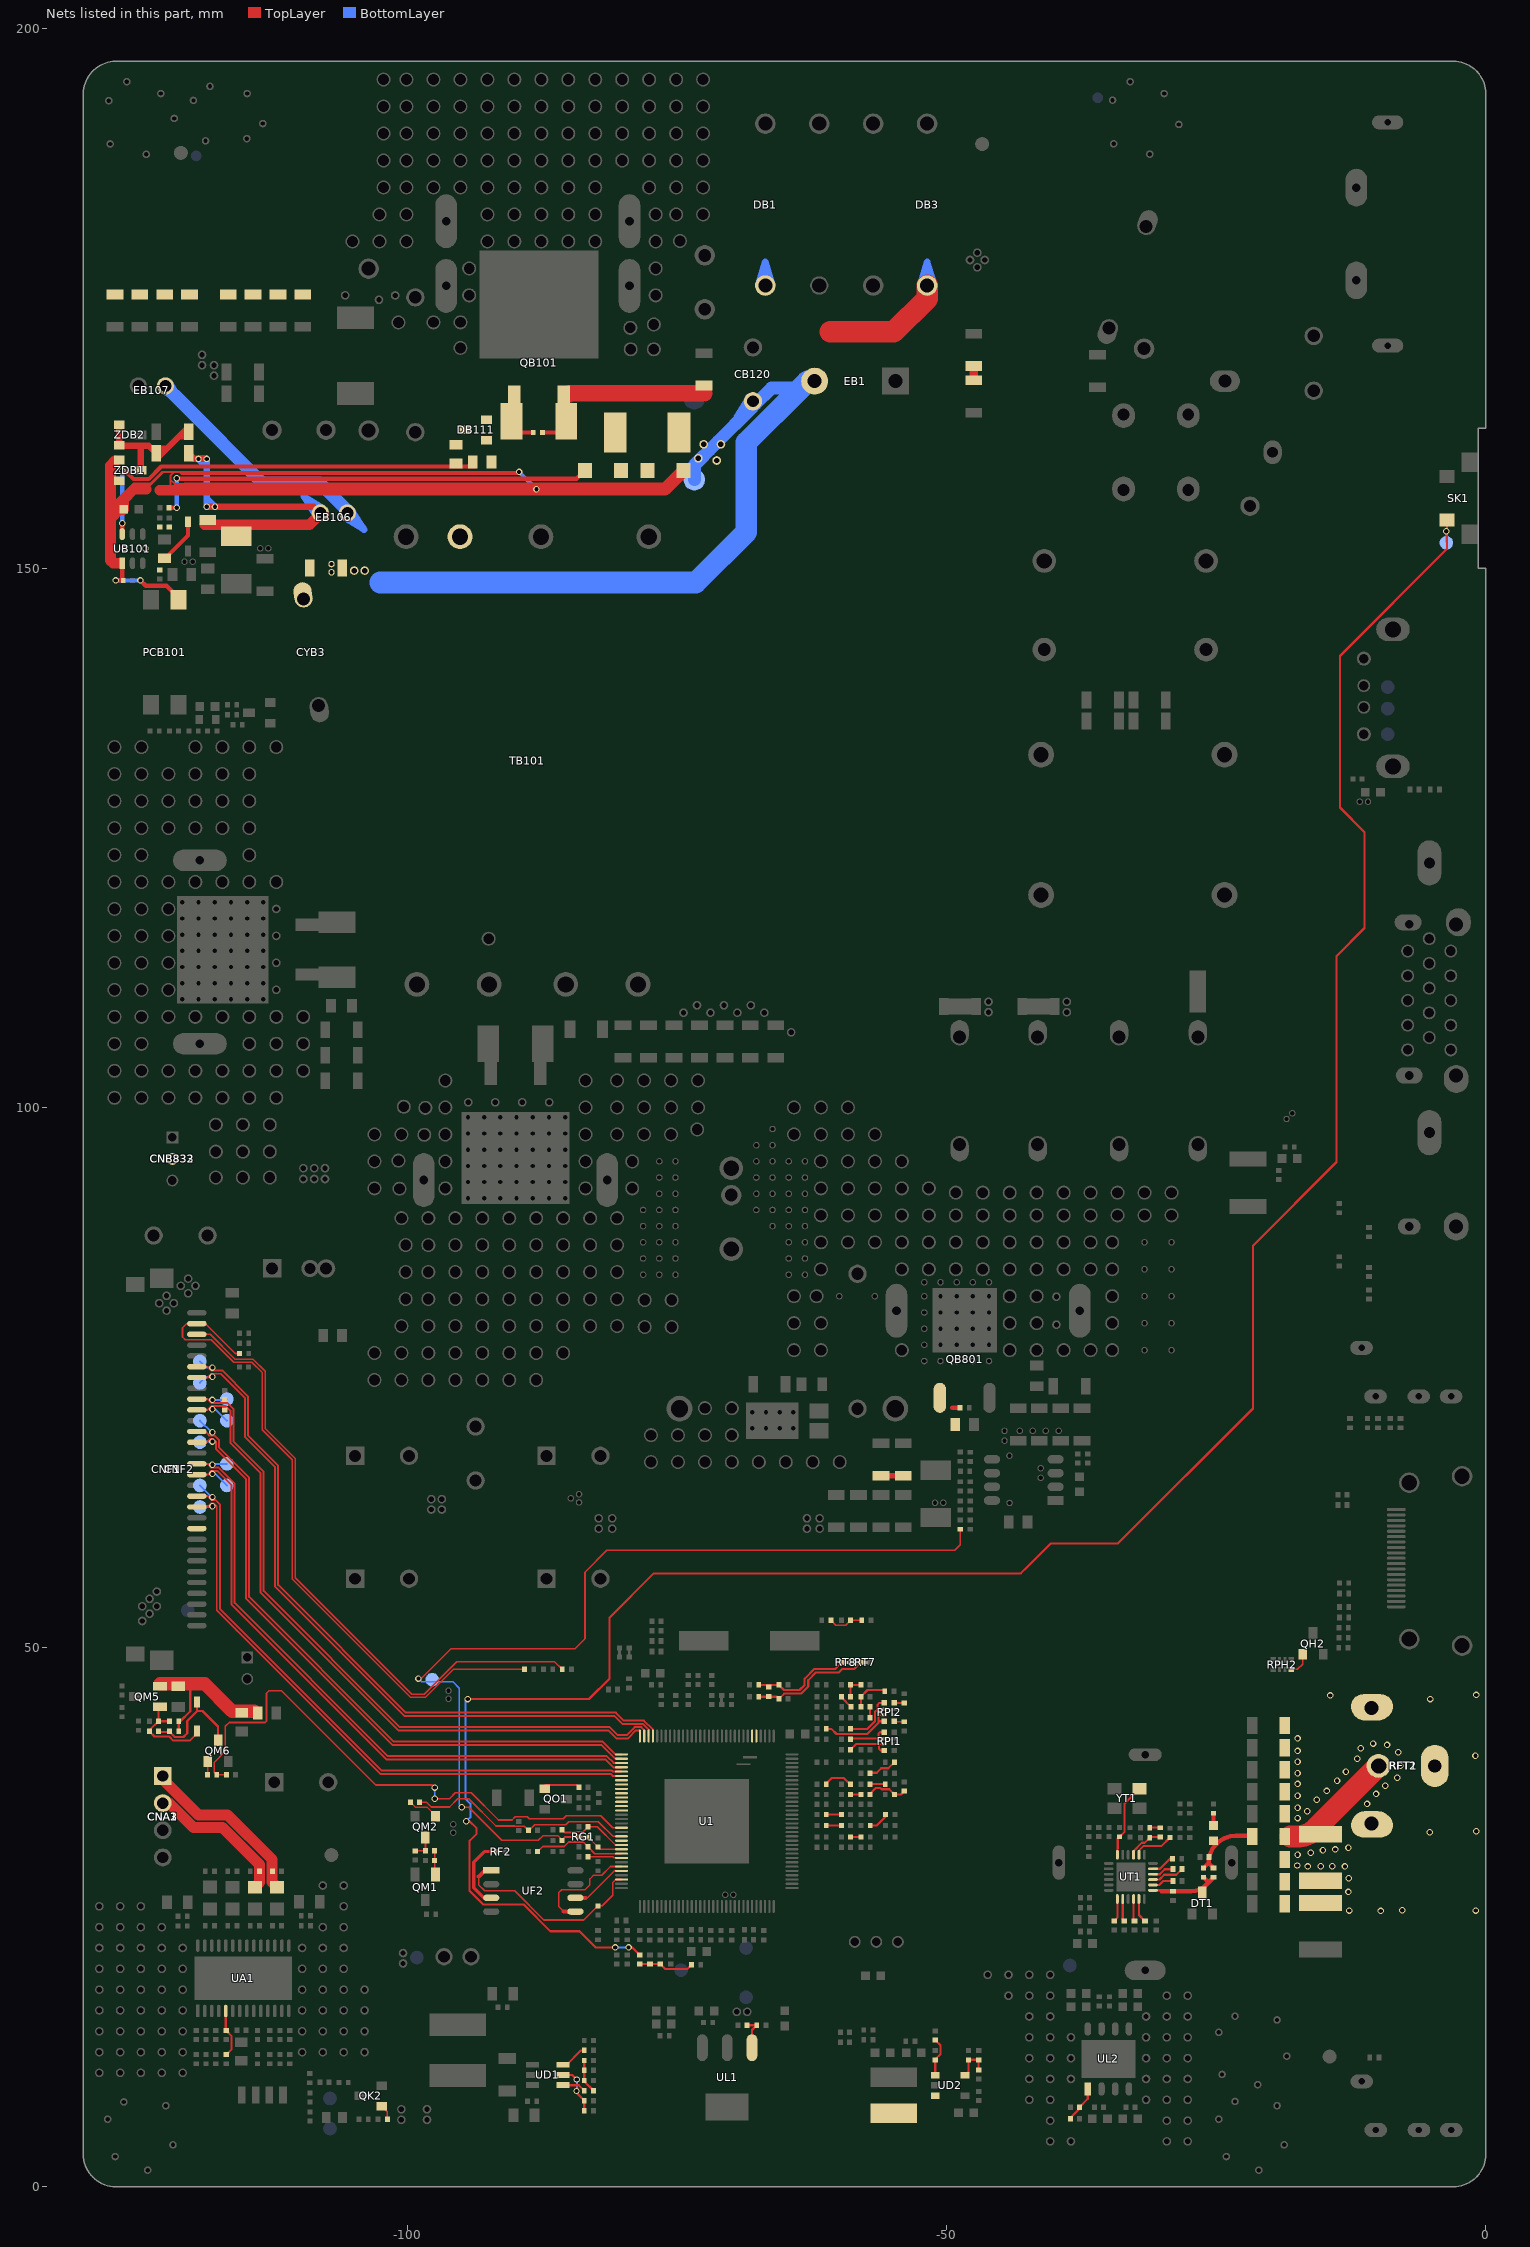
[diagram p0: the nets of this part, all layers, seen from the top]
# Altium PCB MISC84438.PcbDoc (part 12 of 15)
Units mm, origin at the board's own origin, x right, y up, seen from the top; angles counter-clockwise.
Board outline 130 x 197 mm, 2 copper layers (TopLayer, BottomLayer), stack 1.571 mm thick; 574 components, 314 nets, 2636 pads, 811 vias.

## Via types
v1: diameter 0.6, hole 0.4, TopLayer to BottomLayer, tented both sides, 780 vias
v2: diameter 0.7, hole 0.5, TopLayer to BottomLayer, tented both sides, 15 vias
v3: diameter 0.8, hole 0.6, TopLayer to BottomLayer, tented both sides, 12 vias
v4: diameter 0.8, hole 0.5, TopLayer to BottomLayer, tented both sides, 4 vias

## Nets (pads, with @x,y where several pads share a name; then routed paths per layer and width w, separated by ;. In a path a pad name is that pad's centre, name@x,y a point inside that pad or via, vN(x,y) a via of type N, cw(c..) or ccw(c..) an arc to the next point about the centre after c; other vN are vias at no path point) (continued)
NetCD13_2: CD13.2 RD6.1 RD7.2 UD2.5 | length 3.4
  TopLayer w0.203: UD2.5@-48.28,10.335 -47.955,10.66 CD13.2@-47.955,11.754 RD6.1@-47.015,11.754 RD7.2@-47.015,10.814
NetCD17_2: CD17.2 RD8.2 UD2.1 | length 3.7
  TopLayer w0.203: UD2.1@-51.03,10.335 -51.03,11.751 CD17.2@-51.027,11.754 ; RD8.2@-51.027,13.583 -50.548,13.104 -50.548,12.285 -51.027,11.806 CD17.2@-51.027,11.754 ; CD17.2@-50.933,11.754 CD17.2@-51.027,11.754
NetCD20_2: CD20.2 RD13.1 RD15.2 RD16.2 | length 3.1
  TopLayer w0.203: CD20.2@-83.571,11.697 RD13.1@-83.571,10.771 RD16.2@-83.571,9.842 -83.571,9.753 RD15.2@-82.721,8.903
NetCF26_2: CF26.2 RF12.1 | length 2.7
  TopLayer w0.203: CF26.2@-57.081,38.303 -57.014,38.37 -56.464,38.37 -56.052,38.782 -55.383,38.782 RF12.1@-54.82,39.345
NetCF31_2: CF31.2 RF16.1 | length 2
  TopLayer w0.203: CF31.2@-57.055,33.477 -56.464,33.477 -55.632,34.309 RF16.1@-55.632,34.493
NetCF34_1: CF34.1 RF19.2 | length 2.8
  TopLayer w0.203: CF34.1@-61.145,37.312 -61.145,37.369 -60.63,37.883 -59.506,37.883 -58.936,37.313 RF19.2@-58.884,37.313
NetCF39_2: CF39.2 CF40.2 RF24.1 | length 3.2
  TopLayer w0.152: RF24.1@-60.7,52.489 -60.247,52.036 -59.337,52.036 CF39.2@-58.884,52.489 CF40.2@-57.854,52.489
NetCI1_2: CI1.2 RI2.2 | length 1
  TopLayer w0.203: CI1.2@-58.884,36.347 RI2.2@-57.931,36.346
NetCI3_2: CI3.2 RPI2.5 RPI2.7 | length 7.4
  TopLayer w0.198: CI3.2@-61.145,42.431 -60.661,42.431 -60.185,41.955 -59.931,41.955 -57.331,41.955 -56.304,42.981 -56.304,43.167 ; RPI2.7@-55.695,43.143 RPI2.7@-55.746,43.143 -56.28,43.143 -56.304,43.167 ; RPI2.5@-55.695,43.743 RPI2.5@-55.746,43.743 -56.232,43.743 -56.304,43.67 -56.304,43.167
NetCI4_2: CI4.2 RPI2.1 RPI2.3 | length 5.6
  TopLayer w0.198: CI4.2@-58.884,42.431 -57.314,42.431 -56.63,43.115 -56.63,43.993 -56.38,44.243 ; RPI2.3@-55.695,44.243 -56.38,44.243 ; RPI2.1@-55.695,44.843 -56.211,44.843 -56.38,44.674 -56.38,44.243
NetCI6_2: CI6.2 RPI1.5 RPI1.7 | length 4.4
  TopLayer w0.198: CI6.2@-58.884,40.5 -58.359,41.025 -56.236,41.025 ; RPI1.7@-55.746,40.425 -56.097,40.425 -56.236,40.564 -56.236,41.025 ; RPI1.5@-55.695,41.025 RPI1.5@-55.746,41.025 -56.236,41.025
NetCI7_2: CI7.2 RPI1.1 RPI1.3 | length 4
  TopLayer w0.198: -58.621,41.525 -56.312,41.525 ; RPI1.1@-55.746,42.125 -56.173,42.125 -56.312,41.986 -56.312,41.525 ; RPI1.3@-55.695,41.525 RPI1.3@-55.746,41.525 -56.312,41.525
NetCI8_2: CI8.2 RI8.2 | length 1.4
  TopLayer w0.203: CI8.2@-57.081,37.313 RI8.2@-55.67,37.313
NetCM1_2: CM1.2 QM1.G RM2.2 | length 2.1
  TopLayer w0.152: QM1.G@-97.441,29.012 RM2.2@-97.441,31.147
NetCM3_1: CM3.1 CM7.1 DM1.K QM5.G RM7.2 | length 8.9
  TopLayer w0.203: QM5.G@-122.892,44.478 -123.032,44.338 CM7.1@-123.032,43.142 ; CM3.1@-122.003,43.142 CM7.1@-123.032,43.142 ; DM1.K@-119.344,42.124 -120.125,41.343 -121.66,41.343 -122.041,41.724 -123.403,41.724 RM7.2@-123.882,42.202 -123.882,42.292 CM7.1@-123.032,43.142
NetCNB832_2: CNB832.2 CNB833.2
NetCNF1_21: CNF1.21 CNF2.21
NetCO1_1: CO1.1 RO3.2 RO13.2 | length 3.4
  TopLayer w0.203: CO1.1@-57.931,44.475 RO3.2@-57.931,45.416 -57.317,46.029 -55.814,46.029 RO13.2@-55.721,45.936
NetCO1_2: CO1.2 RO1.2 | length 1
  TopLayer w0.198: RO1.2@-57.081,43.459 CO1.2@-57.081,44.475
NetCO4_1: CO4.1 RO7.2 RO15.2 | length 2.1
  TopLayer w0.203: CO4.1@-58.884,45.415 RO7.2@-58.884,46.507 ; RO7.2@-58.844,46.507 RO7.2@-58.884,46.507 ; RO15.2@-57.931,46.507 RO7.2@-58.884,46.507
NetCO4_2: CO4.2 RO5.2 | length 1.3
  TopLayer w0.203: CO4.2@-59.734,45.415 -59.734,45.351 RO5.2@-58.859,44.475
NetCT10_1: CT10.1 CT20.1 RT7.2 RT7.3 RT9.1 | length 11.3
  TopLayer w0.203: CT20.1@-67.4,45.415 -66.453,45.415 -65.735,45.415 CT10.1@-65.532,45.212 -65.046,45.698 -63.481,45.698 -62.814,46.364 -62.814,46.952 -62.116,47.65 -59.992,47.65 -59.666,47.977 -58.544,47.977 RT7.2@-57.931,48.59
NetCT11_2: CT11.2 UT1.20 | length 2.1
  TopLayer w0.203: UT1.20@-33.656,26.664 -33.656,24.754 CT11.2@-33.533,24.631
NetCT12_1: CT12.1 UT1.19 | length 2.2
  TopLayer w0.203: CT12.1@-34.461,24.631 -34.156,24.936 UT1.19@-34.156,26.664
NetCT13_2: CT13.2 DT1.2 LT3.2 LT6.1 UT1.1 | length 6.7
  TopLayer w0.229: UT1.1@-30.856,27.464 -30.107,27.464
  TopLayer w0.401: -30.061,27.387 LT6.1@-28.981,27.387 -27.305,27.387 ccw(c-27.305,29.288) -25.961,27.944 LT3.2@-25.227,28.678 ; CT13.2@-26.167,28.678 -25.705,28.216
NetCT15_2: CT15.2 UT1.12 YT1.3 | length 7
  TopLayer w0.203: UT1.12@-34.156,30.764 -34.156,31.304 -34.116,31.344 -34.116,32.273 CT15.2@-33.96,32.429 -33.481,32.908 -33.481,35.513 YT1.3@-32.115,36.879
NetCT17_1: CT17.1 LT9.2 | length 1.1
  TopLayer w0.401: LT9.2@-25.248,33.485 CT17.1@-25.248,34.614
NetCT21_1: CT21.1 UT1.5 | length 2.2
  TopLayer w0.203: UT1.5@-30.856,29.464 -30.2,29.464 -29.274,30.391 CT21.1@-29.038,30.391
NetCT23_1: CT23.1 CT24.2 RT8.2 RT8.3 RT9.2 | length 9.1
  TopLayer w0.203: CT23.1@-67.4,46.507 -66.453,46.507 -65.532,46.507 -65.053,46.028 -63.618,46.028 -63.144,46.501 -63.144,47.089 -62.253,47.98 -60.314,47.98 RT8.2@-59.875,48.42
NetCT25_1: CT25.1 UT1.8 | length 3.8
  TopLayer w0.191: UT1.8@-32.156,30.764 -32.156,31.149 -31.748,31.557 -30.083,31.557 CT25.1@-29.274,32.366
NetCT26_2: CT26.2 RT11.2 UT1.9 | length 3.3
  TopLayer w0.191: UT1.9@-32.656,30.764 -32.656,31.098 -31.88,31.874 -31.619,31.874 CT26.2@-31.147,32.346 -31.076,32.417 RT11.2@-30.188,32.417
NetCT29_2: CT29.2 RT11.1 | length 1
  TopLayer w0.191: CT29.2@-31.147,33.274 -30.195,33.274 RT11.1@-30.188,33.267
NetCV1_2: CV1.2 RV1.1 | length 1.4
  TopLayer w0.18: CV1.2@-61.145,34.493 RV1.1@-59.734,34.493
NetCV3_2: CV3.2 RV3.1 | length 1.4
  TopLayer w0.18: CV3.2@-61.145,33.477 RV3.1@-59.734,33.477
NetCV7_2: CV7.2 RV9.1 | length 1
  TopLayer w0.18: CV7.2@-58.884,32.41 RV9.1@-57.905,32.41
NetCYB3_1: CYB3.1 RB130.2
NetDB104_K: DB104.K EB106.1 pad.VIA5@-117.805,155.723 pad.VIA5@-118.567,155.723 pad.VIA5@-118.567,160.147 pad.VIA5@-119.329,160.147 RB110.2 RB116.2 | length 33.3
  TopLayer w0.6: RB110.2@-120.242,160.68 -119.709,160.147 pad.VIA5@-119.329,160.147 pad.VIA5@-118.681,160.147 ; pad.VIA5@-118.567,155.723 pad.VIA5@-117.805,155.723 -108.636,155.723 EB106.1@-108.032,155.119
  TopLayer w1: RB116.2@-118.745,154.038 -114.786,154.038 ; DB104.K@-115.83,152.995 -114.786,154.038 ; EB106.1@-108.032,155.038 -109.032,154.038 -114.786,154.038
  BottomLayer w0.6: -118.567,156.485 pad.VIA5@-117.805,155.723 pad.VIA5@-118.567,155.723 -118.567,156.485 ; -118.567,156.485 -118.567,159.385 ; -118.567,159.385 pad.VIA5@-119.329,160.147 pad.VIA5@-118.567,160.147 -118.567,159.385
NetDB109_A: DB109.A QB101.3 RB105.2 RB109.1 RB119.1 RB148.2 | length 56.4
  TopLayer w0.4: RB105.2@-122.054,155.613 v1(-121.336,155.613) ; v1(-121.336,158.344) -121.301,158.308 -84.284,158.308 DB109.A@-83.517,159.075 ; RB109.1@-87.446,162.598 QB101.3@-85.331,162.598
  TopLayer w1.5: QB101.3@-85.051,166.103 -84.924,166.23 -72.415,166.23
  BottomLayer w0.4: v1(-121.336,155.613) v1(-121.336,158.344)
NetDB109_K: DB109.K DB110.A
NetDB111_1: DB111.1 DB111.3 QB101.1 RB106.2 RB109.2 | length 2.1
  TopLayer w0.4: QB101.1@-90.411,162.598 RB109.2@-88.296,162.598
NetDB111_2: DB111.2 RB107.2
NetDB112_K: DB112.K RB112.2 | length 4.3
  TopLayer w0.4: RB112.2@-122.479,151.102 -122.253,151.102 -120.307,153.048 DB112.K@-120.307,154.321
NetDK1_K: DK1.K RK3.2 RK4.1 RK6.1 | length 5.2
  TopLayer w0.203: RK6.1@-78.435,20.629 RK3.2@-76.517,20.629 -76.064,20.175 -74.011,20.175 RK4.1@-73.628,20.559
NetDM1_A: DM1.A QM6.C RM5.1 RM7.1 | length 10.1
  TopLayer w0.203: RM7.1@-123.032,42.202 -122.981,42.151 -122.002,42.151 -121.523,41.673 -120.713,41.673 -120.371,42.016 -120.371,43.167 -119.456,44.082 ; DM1.A@-119.456,44.936 -119.456,44.082 ; QM6.C@-117.513,41.377 -117.513,42.647 -118.948,44.082 -119.456,44.082
NetKEY_1: KEY.1 RK6.2 SK1.2 | length 217.2
  TopLayer w0.203: v1(-94.501,33.871) -94.208,33.871 -93.548,33.211 -93.548,32.715 -94.196,32.067 -94.196,27.407 -92.951,26.162 -89.193,26.162 -86.708,23.678 -84.015,23.678 -82.512,22.174 v1(-80.709,22.174) ; v1(-94.374,45.199) -83.121,45.199 -81.216,47.104 -81.216,52.755 -77.126,56.845 -43.103,56.845 -42.462,57.486 -40.334,59.614 -34.111,59.614 -21.59,72.135 -21.59,87.223 -13.843,94.97 -13.843,114.062 -11.239,116.665 -11.239,125.549 -13.525,127.835 -13.525,141.887 -3.603,151.81 SK1.2@-3.603,154.5 ; v1(-79.464,22.174) -79.131,22.174 RK6.2@-78.435,21.479
  BottomLayer w0.203: v1(-94.501,33.871) -94.125,34.247 -94.125,35.501 -94.577,35.953 -94.577,44.996 v1(-94.374,45.199) ; v1(-80.709,22.174) v1(-79.464,22.174) ; KEY.1@-3.658,152.476 v1(-3.658,153.441)
NetLD2_1: LD2.1 UD2.3
NetLT1_2: LT1.2 UT1.23 | length 2.3
  TopLayer w0.203: UT1.23@-32.156,26.664 -32.156,25.176 LT1.2@-31.61,24.631
NetLT2_1: LT2.1 UT1.22 | length 2
  TopLayer w0.203: LT2.1@-32.656,24.711 UT1.22@-32.656,26.664
NetLT8_1: LT8.1 UT1.2 | length 2
  TopLayer w0.203: UT1.2@-30.856,27.964 -30.278,27.964 -29.922,28.32 LT8.1@-29.012,28.32
NetLT10_1: LT10.1 UT1.4 | length 2
  TopLayer w0.203: UT1.4@-30.856,28.964 -30.215,28.964 -29.754,29.425 LT10.1@-29.012,29.425
NetLT10_2: LT10.2 UT1.3 | length 3.1
  TopLayer w0.203: UT1.3@-30.856,28.464 -30.248,28.464 -29.807,28.905 -28.683,28.905 LT10.2@-28.162,29.425
NetQB801_G: QB801.G RB807.2 RB808.2 | length 0.7
  TopLayer w0.4: -49.466,72.2 RB808.2@-48.736,72.2
NetQH2_B: QH2.B RPH2.7 | length 2.2
  TopLayer w0.127: RPH2.7@-18.022,47.937 -17.468,47.937 -16.98,48.425 QH2.B@-16.98,49.352
NetQK2_B: QK2.B RK20.1 | length 2
  TopLayer w0.152: QK2.B@-102.349,7.455 -101.823,6.928 RK20.1@-101.823,6.248 -101.823,6.839
NetQM2_B: QM2.B RM4.1 | length 2.8
  TopLayer w0.152: RM4.1@-99.688,35.636 -99.235,35.183 -98.14,35.183 QM2.B@-97.358,34.401
NetQM2_C: QM2.C RM1.1 RM2.1 | length 2.2
  TopLayer w0.152: RM1.1@-99.238,31.115 -99.206,31.147 RM2.1@-98.291,31.147 -98.291,32.321 QM2.C@-98.323,32.353
NetQM6_B: QM6.B RM8.2 | length 1.2
  TopLayer w0.152: RM8.2@-118.484,38.176 -118.484,39.389 QM6.B@-118.478,39.395
NetQO1_B: QO1.B RO10.1 | length 3.2
  TopLayer w0.152: QO1.B@-87.211,37.223 -84.283,37.223 RO10.1@-84.067,37.007
NetRA4_1: RA4.1 RA14.2 UA1.5 | length 4.5
  TopLayer w0.203: UA1.5@-116.8,16.29 -116.8,14.545 RA14.2@-116.737,14.482 -116.737,14.43 -116.259,13.951 -116.259,12.725 RA4.1@-116.737,12.247
NetRB101_2: RB101.2 RB102.1 | length 1.3
  TopLayer w0.762: RB102.1@-47.473,167.438 RB101.2@-47.473,168.756
NetRB106_1: RB106.1 RB107.1 UB101.6 | length 40
  TopLayer w0.4: v1(-126.403,154.191) -126.4,154.188 UB101.6@-126.4,153.177 ; v1(-126.403,159.055) -126.111,159.055 -125.349,158.293 -123.927,158.293 -122.781,159.439 RB106.1@-94.348,159.439 ; RB106.1@-93.906,159.88 RB106.1@-94.348,159.439 ; RB106.1@-93.738,159.439 RB106.1@-94.348,159.439
  BottomLayer w0.4: v1(-126.403,154.191) v1(-126.403,159.055)
NetRB110_1: RB110.1 RB111.2 ZDB1.2 ZDB2.1 ZDB2.3 | length 14.1
  TopLayer w0.6: ZDB2.1@-126.67,163.28 ZDB2.3@-126.67,161.417 -126.67,161.375 -123.937,161.375 RB110.1@-123.242,160.68 ; ZDB1.2@-124.688,159.093 -124.688,161.351 ; RB110.1@-123.304,160.68 RB110.1@-123.242,160.68 ; RB110.1@-123.101,160.261 -122.276,161.087 ; RB111.2@-120.282,163.081 -121.107,162.255 ; RB111.2@-120.242,162.655 -120.642,162.255 -121.107,162.255 ; RB110.1@-123.242,160.68 -122.836,161.087 -122.276,161.087 ; -122.276,161.087 -121.107,162.255
NetRB150_1: RB150.1 RB151.1 RB152.1 RB153.2 RB154.2 RB155.2 RB156.1 RB157.2
NetRB814_2: RB814.2 RB835.1 | length 2.1
  TopLayer w0.5: RB814.2@-56.069,65.899 RB835.1@-53.993,65.899
NetRD2_1: RD2.1 UD1.6 | length 2.5
  TopLayer w0.203: UD1.6@-85.556,11.301 -85.206,11.301 -83.883,12.625 RD2.1@-83.571,12.625
NetRD14_2: RD14.2 RD88.2 UD1.5 | length 4.8
  TopLayer w0.203: UD1.5@-85.556,10.351 -84.672,10.351 v1(-84.252,9.931) ; v1(-84.29,8.865) -84.29,8.696 RD88.2@-83.571,7.977 ; RD14.2@-83.571,7.048 RD88.2@-83.571,7.977 ; RD88.2@-83.571,7.898 RD88.2@-83.571,7.977
  BottomLayer w0.203: v1(-84.29,8.865) -84.252,8.903 v1(-84.252,9.931)
NetRD15_1: RD15.1 UD1.4 | length 2.2
  TopLayer w0.203: UD1.4@-85.556,9.401 -84.069,9.401 RD15.1@-83.571,8.903
NetRF2_1: RF2.1 UF2.3 | length 6.7
  TopLayer w0.305: UF2.3@-92.19,26.772 -92.888,26.772 -93.815,27.699 -93.815,30.074 -92.825,31.064 RF2.1@-91.91,31.064
NetRI2_1: RI2.1 RI3.2 RI14.2 | length 3.9
  TopLayer w0.203: RI2.1@-57.081,36.346 -57.081,36.428 -56.566,36.942 -56.098,36.942 -55.99,36.834 -55.307,36.834 RI3.2@-54.82,36.347 ; RI3.2@-54.781,36.347 RI3.2@-54.82,36.347 ; RI14.2@-53.899,36.659 -54.211,36.347 RI3.2@-54.82,36.347
NetRI13_2: RI13.2 RPI2.2 | length 0.9
  TopLayer w0.203: RPI2.2@-54.846,44.843 -54.84,44.837 RI13.2@-53.899,44.837
NetRI15_2: RI15.2 RPI2.8 | length 1
  TopLayer w0.152: RPI2.8@-54.846,43.143 -54.8,43.097 RI15.2@-53.899,43.097
NetRL1_2: RL1.2 RL2.1 UL1.1 | length 3.2
  TopLayer w0.203: RL1.2@-68.485,14.961 RL2.1@-67.583,14.961 -68.023,14.52 UL1.1@-68.023,12.877
NetRL4_2: RL4.2 RL5.1 UL2.1 | length 3.4
  TopLayer w0.203: RL5.1@-38.512,6.299 -38.512,6.37 -37.662,7.22 RL4.2@-37.662,7.367 -36.893,8.135 UL2.1@-36.893,9.054
PANEL_ON/OFF: RM8.1 RM10.1 U1.82 | length 52.4
  TopLayer w0.152: RM10.1@-116.706,38.176 RM10.1@-116.732,38.176 RM8.1@-117.634,38.176 -117.875,38.417 -117.875,39.311 -116.839,40.347 -116.839,42.673 -116.484,43.028 -113.132,43.028 -113.03,43.129 -113.03,45.72 -112.789,45.961 -111.632,45.961 -102.894,37.223 -97.65,37.223 v1(-97.422,36.995) ; v1(-97.422,35.966) -96.061,35.966 -95.515,36.512 -94.047,36.512 -91.52,33.985 -90.265,33.985 -89.971,34.28 -88.84,34.28 -88.664,34.103 -85.52,34.103 -85.231,34.393 -82.046,34.393 -80.924,33.271 U1.82@-80.112,33.271
  BottomLayer w0.152: v1(-97.422,35.966) v1(-97.422,36.995)
PC_LIN: U1.38
PC_RIN: U1.37
PVCC: CM3.2 CM5.2 QM5.S R5V.2 R12V.2 RM5.2 | length 14.2
  TopLayer w0.203: RM5.2@-121.152,42.151 RM5.2@-121.152,42.202 -121.152,43.116 -121.035,43.116 -120.091,44.061 -120.091,46.076
  TopLayer w1.27: QM5.S@-122.872,46.609 -118.745,46.609 -116.207,44.071 R5V.2@-114.173,44.071
PWM0: R1.1 R3.1 U1.86 | length 6.5
  TopLayer w0.152: R3.1@-85.63,33.071 -85.381,32.822 -84.418,32.822 -84.343,32.897 -83.67,32.897 R1.1@-83.217,33.35 -82.359,33.35 -80.68,31.671 U1.86@-80.112,31.671
PWM1: R2.1 RG1.1 U1.87 | length 3.6
  TopLayer w0.152: RG1.1@-83.217,32.41 -82.296,31.489 R2.1@-82.296,31.477 -82.089,31.271 U1.87@-80.112,31.271
PWM_REF: CG1.1 PWM_REF.1 RB813.2 RG1.2 RG1.3 | length 88.3
  TopLayer w0.152: v1(-98.941,47.099) -98.685,47.099 -95.923,49.86 -84.431,49.86 -83.502,50.789 -83.502,56.961 -81.475,58.989 -49.241,58.989 -48.73,59.499 RB813.2@-48.73,60.941 ; v1@-94.958,35.166 v1(-94.932,35.166) -94.282,35.166 -91.221,32.106 -87.833,32.106 -87.401,32.538 -86.012,32.538 -85.63,32.156 -85.376,32.41 RG1.2@-84.067,32.41
  BottomLayer w0.152: v1(-98.941,47.099) -98.629,46.787 -97.663,46.787 -95.741,46.787 -95.161,46.207 -95.161,35.369 v1@-94.958,35.166
PWR_ON/OFF: RM3.2 RM4.2 U1.84 | length 21.3
  TopLayer w0.127: -90.03,33.426 -89.122,33.426 RM3.2@-88.741,33.045
  TopLayer w0.152: RM4.2@-98.838,35.636 -98.198,35.636 -97.746,35.184 -96.053,35.184 -95.284,35.953 -94.279,35.953 -91.752,33.426 -90.03,33.426 ; RM3.2@-88.741,33.045 -88.654,33.045 -88.155,33.544 -85.289,33.544 -84.999,33.834 -82.278,33.834 -80.914,32.471 U1.84@-80.112,32.471
REMOTE: CK6.2 RK16.1 U1.88 | length 8.6
  TopLayer w0.152: RK16.1@-87.891,31.064 -87.428,31.526 -85.422,31.526 -84.999,31.949 -83.67,31.949 CK6.2@-83.217,31.496 -82.592,30.871 U1.88@-80.112,30.871
RESET-H: RR1.2 U1.89 | length 3.2
  TopLayer w0.152: RR1.2@-83.217,30.591 -80.924,30.591 -80.804,30.471 U1.89@-80.112,30.471
RF_IN: CT40.1 GDT1.1 RFT1.1 RFT2.1 | length 10.8
  TopLayer w2.032: -18.11,32.45 -17.552,32.45 ccw(c-17.552,34.99) -15.756,33.194 RFT2.1@-9.95,39
RF_INPUT: CT13.1 CT40.2 LT3.1 LT9.1 LT11.1 | length 6.8
  TopLayer w0.401: CT13.1@-26.167,29.528 -25.705,29.99 ; -25.697,29.99 cw(c-23.163,29.99) -25.697,29.998 ; LT3.1@-25.227,29.528 -25.697,29.998 ; CT40.2@-21.642,32.524 -23.163,32.524 ccw(c-23.163,29.99) -25.697,29.998
RFGND: CT41.2 CT42.2 CT43.2 CT44.2 CT45.2 CT46.2 CT47.2 CT48.2 GDT1.2 GDT2.2 RFT1.2 RFT1.3 RFT1.4 RFT2.2 RFT2.3 RFT2.4
  other v1: -9.741,25.552 -12.649,25.59 -0.94,25.59 -7.76,25.616 -12.738,27.318 -12.713,28.588 -16.497,29.68 -13.056,29.68 -15.316,29.705 -14.237,29.705 -17.488,29.769 -17.45,30.759 -16.243,30.95 -15.1,31.191 -13.957,31.255 -12.738,31.407 -5.194,32.855 -0.876,32.944 -17.45,34.163 -16.561,34.811 -17.45,35.128 -11.011,35.471 -15.659,35.865 -17.45,36.246 -10.173,36.398 -14.732,36.678 -9.335,37.173 -17.45,37.325 -13.792,37.63 -8.217,37.91 -17.45,38.316 -12.967,38.468 -7.938,39.027 -17.45,39.395 -11.913,39.649 -0.965,39.954 -8.128,40.272 -17.45,40.386 -11.595,40.64 -9.157,40.945 -10.452,41.072 -17.45,41.542 -5.156,45.199 -14.427,45.529 -0.876,45.58
ROUT+: CA17.2 CNA1.1 CNA2.1 CNA3.1 LBA4.2 | length 16.3
  TopLayer w1.016: CNA2.1@-122.636,38.07 -122.636,37.754 -119.325,34.442 -116.629,34.442 -112.53,30.344 -112.53,28.229 LBA4.2@-112.051,27.749
ROUT-: CA10.1 CNA1.2 CNA2.2 CNA3.2 LBA3.2 | length 13.6
  TopLayer w1.016: CNA2.2@-122.636,35.55 -122.049,35.55 -119.798,33.299 -117.103,33.299 -113.673,29.87 -113.673,28.185 LBA3.2@-114.108,27.749
RXE0+: CNF1.18 CNF2.18 E0P.1 U1.69 | length 57.2
  TopLayer w0.178: CNF2.18@-119.486,64 -118.488,64 -118.141,63.652 -117.78,63.652 -117.329,63.201 -117.329,53.543 -102.342,38.557 -81,38.557 -80.914,38.471 U1.69@-80.112,38.471
  BottomLayer w0.178: E0P.1@-119.2,65 -118.122,63.922 v1(-118.036,63.922)
RXE0-: CNF1.19 CNF2.19 E0N.1 U1.70 | length 56.8
  TopLayer w0.178: CNF2.19@-119.486,63 -118.488,63 -118.141,63.348 -117.906,63.348 -117.633,63.075 -117.633,53.417 -115.786,51.57 -102.468,38.252 -81.127,38.252 -80.945,38.071 U1.70@-80.112,38.071
  BottomLayer w0.178: E0N.1@-119.2,63 -119.137,63.063 v1(-118.036,63.063)
RXE1+: CNF1.15 CNF2.15 E1P.1 U1.67 | length 58.7
  TopLayer w0.178: CNF2.15@-119.486,67 -118.488,67 -118.141,66.652 -117.467,66.652 -115.982,65.168 -115.982,54.101 -101.784,39.903 -81.484,39.903 -80.852,39.271 U1.67@-80.112,39.271
  BottomLayer w0.178: v1(-118.036,66.922) -117.958,67 E1P.1@-116.7,67
RXE1-: CNF1.16 CNF2.16 E1N.1 U1.68 | length 59.2
  TopLayer w0.178: CNF2.16@-119.486,66 -118.488,66 -118.141,66.348 -117.593,66.348 -116.287,65.042 -116.287,53.975 -101.911,39.598 -81.611,39.598 -80.883,38.871 U1.68@-80.112,38.871
  BottomLayer w0.178: v1(-118.036,66.063) -117.763,66.063 E1N.1@-116.7,65
RXE2+: CNF1.12 CNF2.12 E2P.1 U1.65 | length 60.3
  TopLayer w0.178: CNF2.12@-119.486,70 -118.719,70 -118.351,69.632 -117.866,69.632 -117.416,69.182 -117.416,68.506 -114.636,65.725 -114.636,54.659 -101.227,41.249 -81.86,41.249 -80.682,40.071 U1.65@-80.112,40.071
  BottomLayer w0.178: E2P.1@-119.2,71 -118.122,69.922 v1(-118.036,69.922)
RXE2-: CNF1.13 CNF2.13 E2N.1 U1.66 | length 59.9
  TopLayer w0.178: CNF2.13@-119.486,69 -118.586,69 -118.26,69.327 -117.992,69.327 -117.721,69.056 -117.721,68.379 -117.3,67.959 -114.941,65.599 -114.941,54.532 -101.353,40.945 -81.987,40.945 -80.713,39.671 U1.66@-80.112,39.671
  BottomLayer w0.178: E2N.1@-119.2,69 -119.137,69.063 v1(-118.036,69.063)
RXE3+: CNF1.6 CNF2.6 E3P.1 U1.61 | length 66.8
  TopLayer w0.178: CNF2.6@-119.486,76 -118.488,76 -118.223,75.735 -118.141,75.652 -118.036,75.652 -117.144,75.652 -114.724,73.232 -114.724,69.621 -111.944,66.841 -111.944,55.774 -100.112,43.942 -80.647,43.942 -79.91,43.205 -78.037,43.205 -77.212,42.38 U1.61@-77.212,41.771
  BottomLayer w0.178: E3P.1@-119.2,76.5 -118.622,75.922 v1(-118.036,75.922)
RXE3-: CNF1.7 CNF2.7 E3N.1 U1.62 | length 66.3
  TopLayer w0.178: CNF2.7@-119.486,75 -118.488,75 -118.231,75.258 -118.141,75.348 -118.036,75.348 -117.27,75.348 -115.029,73.106 -115.029,69.495 -112.249,66.714 -112.249,55.648 -100.238,43.637 -80.773,43.637 -80.037,42.901 -78.164,42.901 -77.612,42.349 U1.62@-77.612,41.771
  BottomLayer w0.178: E3N.1@-119.2,74.5 -118.637,75.063 v1(-118.036,75.063)
RXEC+: CF35.2 CNF1.9 CNF2.9 ECP.1 U1.63 | length 64.9
  TopLayer w0.178: CNF2.9@-119.486,73 -118.488,73 -118.141,72.652 -116.661,72.652 -116.07,72.062 -116.07,69.063 -113.29,66.283 -113.29,55.216 -100.669,42.596 -81.204,42.596 -80.468,41.859 -79.628,41.859 -78.901,42.587 -78.281,42.587 -78.012,42.318 U1.63@-78.012,41.771
  BottomLayer w0.178: v1(-118.036,72.922) -116.778,72.922 ECP.1@-116.7,73
RXEC-: CF33.2 CNF1.10 CNF2.10 ECN.1 U1.64 | length 64.7
  TopLayer w0.178: CNF2.10@-119.486,72 -118.488,72 -118.141,72.348 -116.787,72.348 -116.375,71.935 -116.375,68.937 -113.595,66.157 -113.595,55.09 -100.796,42.291 -81.331,42.291 -80.594,41.554 -79.502,41.554 -78.775,42.282 -78.511,42.282 -78.412,42.183 U1.64@-78.412,41.771
  BottomLayer w0.178: v1(-118.036,72.063) -117.763,72.063 ECN.1@-116.7,71
RXO0+: U1.77
RXO0-: U1.78
RXO1+: U1.75
RXO1-: U1.76
RXO2+: U1.73
RXO2-: U1.74
RXO3+: U1.71
RXO3-: U1.72
SCL//WP: CNF1.2 CNF2.2 RF23.2 RF26.2 | length 63.7
  TopLayer w0.152: RF26.2@-115.518,77.229 -115.931,77.229 -118.702,80 CNF2.2@-119.486,80 -120.411,80 -120.807,79.604 -120.807,78.753 -120.566,78.511 -118.153,78.511 -116.067,76.425 -114.384,76.425 -113.416,75.457 -113.416,70.163 -110.636,67.382 -110.636,56.316 -99.684,45.364 -98.283,45.364 -95.693,47.955 RF23.2@-89.096,47.955
SDA: CNF1.3 CNF2.3 RF27.2 | length 58.8
  TopLayer w0.152: CNF2.3@-119.486,79 -118.247,79 -115.951,76.704 -114.268,76.704 -113.136,75.573 -113.136,70.278 -110.356,67.498 -110.356,56.431 -99.569,45.644 -98.399,45.644 -95.381,48.662 -86.324,48.662 RF27.2@-85.617,47.955
SGND: CB101.2 CB102.2 CB103.2 CB120.1 DB1.A DB3.A DB110.K EB1.2 EB106.2 EB107.2 pad.VIA5@-70.9,161.5 pad.VIA5@-71.3,160 pad.VIA5@-72.5,161.5 pad.VIA5@-73,160.2 pad.VIA5@-103.932,149.801 pad.VIA5@-104.897,149.801 pad.VIA5@-107,149.638 pad.VIA5@-107,150.4 pad.VIA5@-124.257,151.841 pad.VIA5@-126.263,151.841 PCB101.3 RB103.1 RB104.1 RB130.1 RB148.1 TB101.4 TP-TDT.2 UB101.1 ZDB1.1 ZDB1.3 | length 224.3
  TopLayer w0.178: -125.832,157.378 -125.333,157.877 -123.754,157.877 -122.685,158.947 -122.562,158.947 ; -124.511,157.734 -123.774,157.734 ; -124.231,157.277 -124.179,157.329 -123.774,157.734 ; -121.928,157.531 -121.928,158.206 ; -120.833,158.835 -120.944,158.947 ; -120.766,158.724 -120.879,158.724 -121.101,158.947 ; -120.139,158.947 -120.944,158.947 ; -119.736,157.353 -120.21,157.828 -121.549,157.828 -121.928,158.206 ; -123.774,157.734 -122.562,158.947 ; -122.562,158.947 -121.57,158.947 ; -121.928,158.206 -121.928,158.589 -121.57,158.947 ; -121.57,158.947 -121.101,158.947 ; -121.101,158.947 -120.944,158.947
  TopLayer w0.4: v1@-126.987,148.882 CB103.2@-126.307,148.882 -126.4,148.975 UB101.1@-126.4,150.477 ; v1(-124.71,148.882) -124.214,148.387 -122.301,148.387 -121.18,147.266 PCB101.3@-121.18,147.107 ; -120.833,158.835 -89.716,158.835 v1(-89.611,158.94) ; EB1.2@-62.58,167.359 EB1.2@-62.208,167.359
  TopLayer w1: ZDB1.1@-127.076,159.944 -127.495,159.525 -127.495,158.14 -127.495,155.169 ; UB101.1@-126.632,150.477 -127.236,150.477 -127.495,150.736 -127.495,154.61 ; -124.179,157.329 -125.335,157.329 -126.271,156.393 ; -122.911,157.253 -120.623,157.253 -120.523,157.353 ; -127.495,154.61 -127.495,155.169 ; -127.495,154.61 -126.632,155.473 CB102.2@-126.271,155.473 -126.271,156.393 ; -127.495,155.169 -126.731,155.933 -126.271,156.393
  TopLayer w1.2: -120.523,157.353 -119.736,157.353 -88,157.353 -76.075,157.353 DB110.K@-74.353,159.075
  TopLayer w2: -60.767,171.933 -54.866,171.933 -51.788,175.01 DB3.A@-51.788,176.222
  BottomLayer w0.4: v1(-126.987,148.882) v1(-124.71,148.882) ; v1(-89.611,158.94) v1(-88,157.329)
  BottomLayer w1.2: EB107.2@-122.402,166.916 -120.846,165.36 -113.386,157.9 -108.065,157.9 EB106.2@-105.532,155.366 ; TP-TDT.2@-73.368,158.226 -73.368,159.568 -72.868,160.068 -71.968,160.968 -71.168,161.768 -68.182,164.754 -67.693,165.243 -66.223,166.713 -63.513,166.713 ; EB1.2@-62.945,167.28 -62.286,167.28 EB1.2@-62.208,167.359
  BottomLayer w2: -102.489,148.692 -73.228,148.692 -68.555,153.365 -68.555,161.671 -63.513,166.713 -62.945,167.28 -62.867,167.359 EB1.2@-62.208,167.359
SPDIF_OUT: U1.85
SPI_CLK: U1.92 UF2.6 | length 5.3
  TopLayer w0.152: -83.439,26.772 -83.261,26.772 -80.762,29.271 U1.92@-80.112,29.271
  TopLayer w0.381: UF2.6@-84.39,26.772 -83.439,26.772
SPI_CSN: RF3.1 U1.94 UF2.1 | length 19
  TopLayer w0.152: -93.345,28.753 -93.345,27.965 -92.799,27.419 -90.019,27.419 -87.319,24.719 -83.605,24.719 RF3.1@-82.296,26.028 -81.899,26.028 -80.924,27.003 -80.924,28.188 -80.642,28.471 U1.94@-80.112,28.471
  TopLayer w0.381: -93.345,28.753 -92.786,29.312 UF2.1@-92.19,29.312
SPI_DI: U1.91 UF2.5 | length 10.2
  TopLayer w0.152: -85.471,25.502 -85.928,25.959 -85.928,27.267 -85.666,27.529 -83.507,27.529 -83.045,27.991 -83.045,28.524 -82.717,28.852 -82.187,28.852 -81.962,28.852 -81.144,29.671 U1.91@-80.112,29.671
  TopLayer w0.381: -85.471,25.502 UF2.5@-84.39,25.502